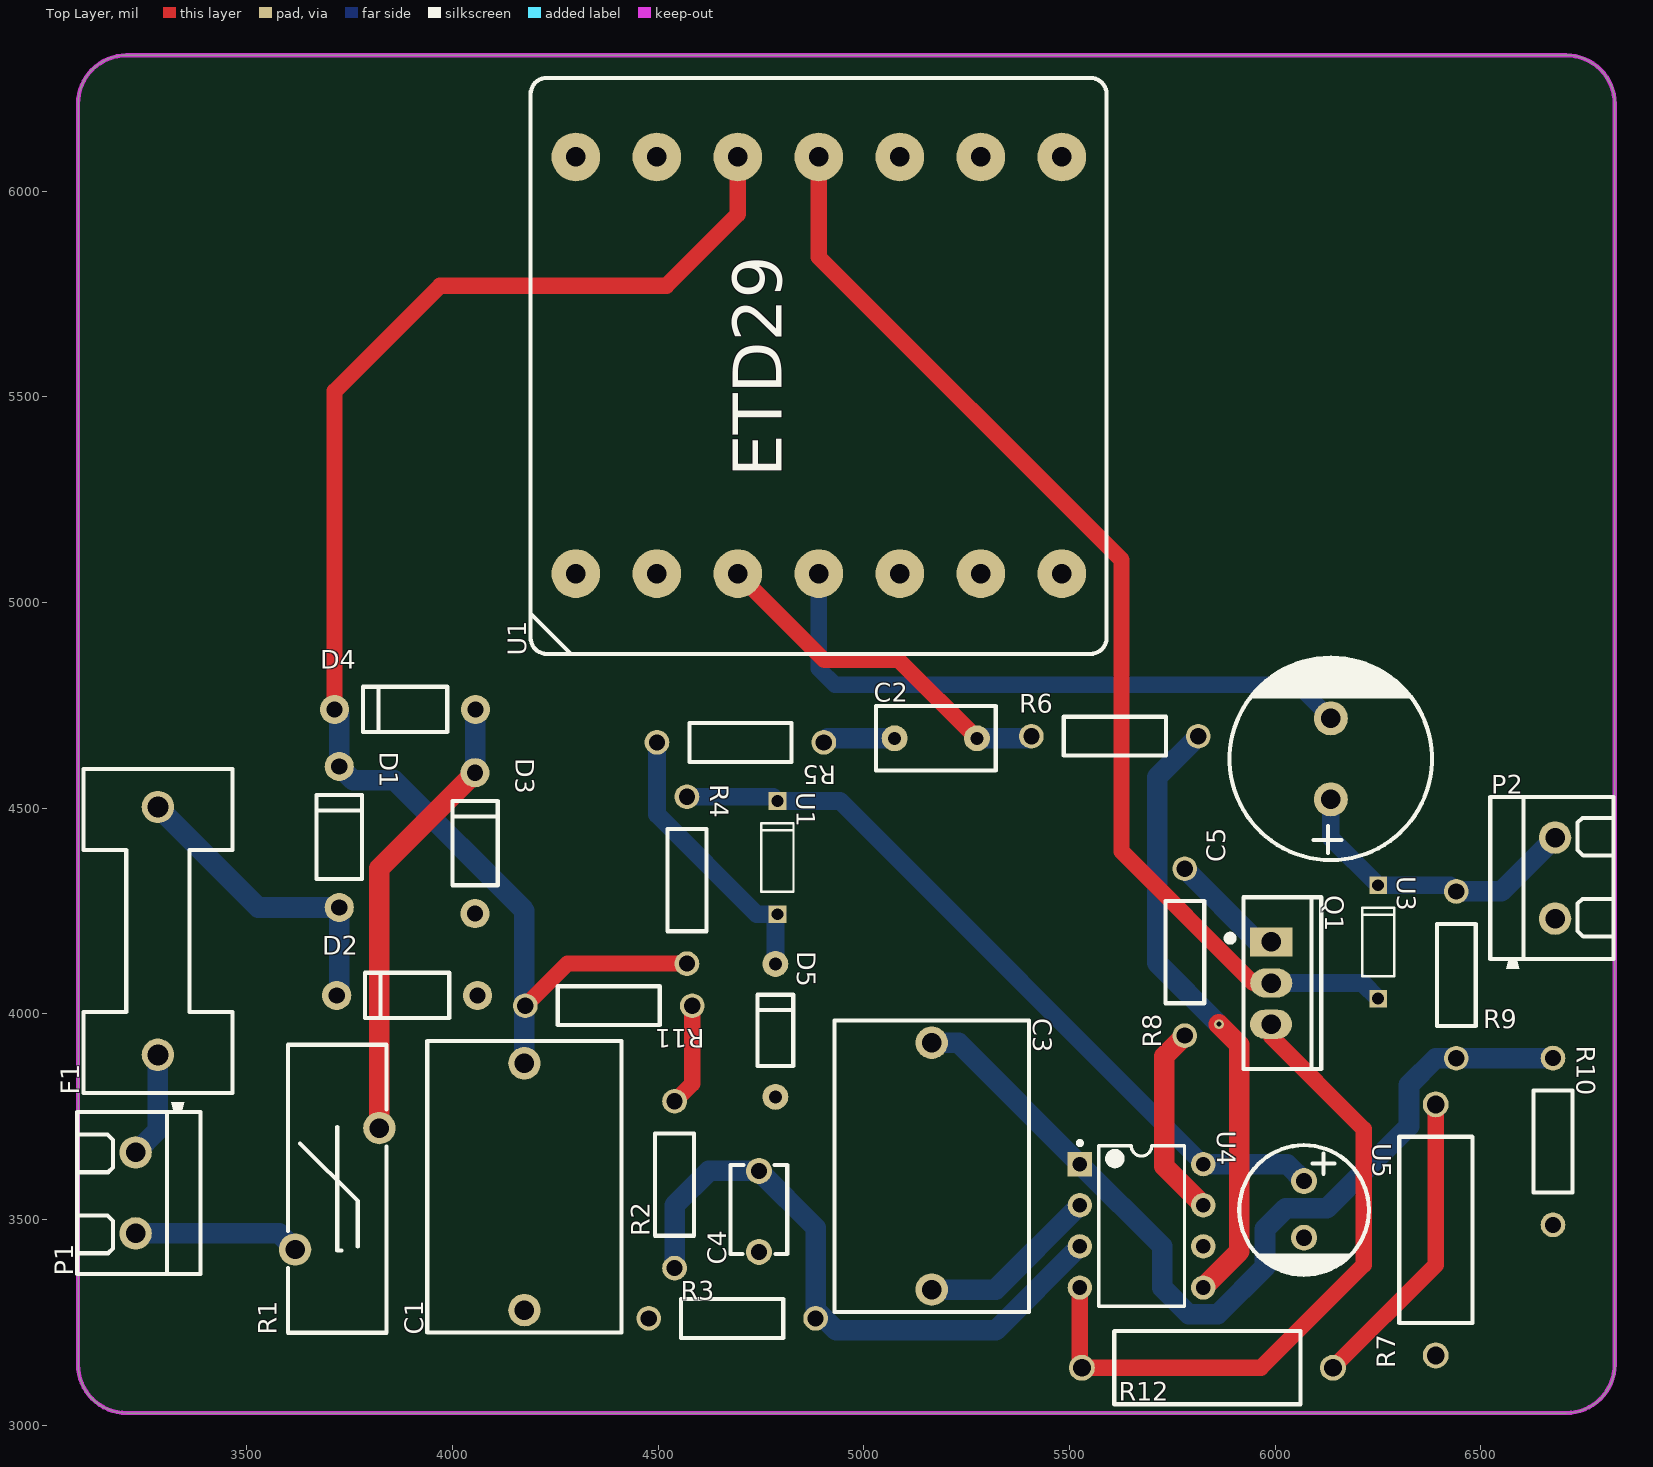
[diagram p0: Top Layer view]
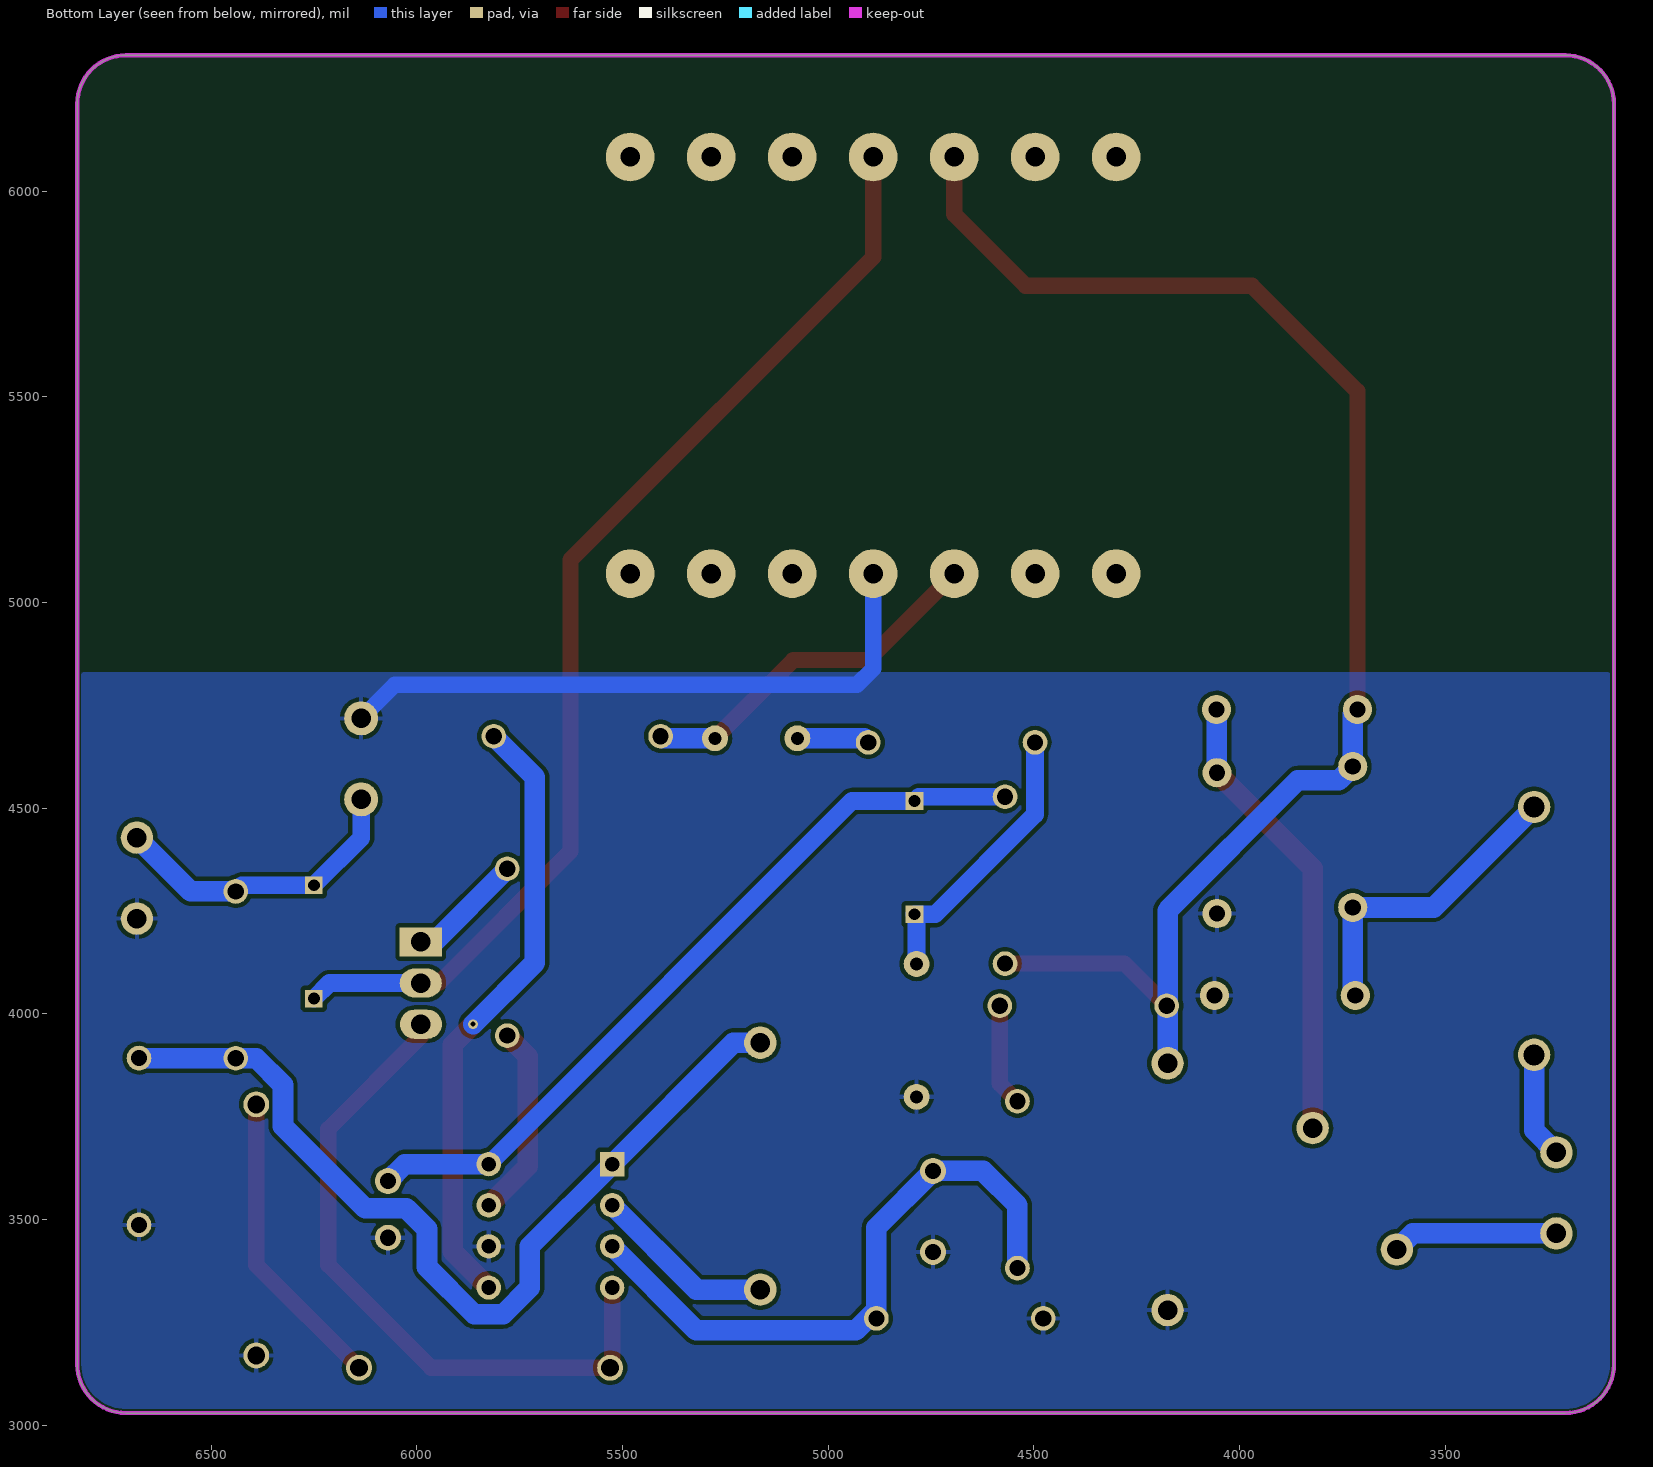
[diagram p1: Bottom Layer view, seen from below]
# Altium PCB MISC89005.pcbdoc
Units mil, origin at the board's own origin, x right, y up, seen from the top; angles counter-clockwise.
Board outline 3735 x 3300 mil, 2 copper layers (Top Layer, Bottom Layer), stack 62.206 mil thick; 31 components, 21 nets, 81 pads, 1 vias.

## Layer stack, top to bottom
Top Solder Mask Layer: solder mask 0.394, Dk 3.3
Top Layer: signal copper 1.379
Dielectric1: surface 59.449, FR4, Dk 4.5
Bottom Layer: signal copper 1.378
Bottom Solder Mask Layer: solder mask 0.394, Dk 3.3

## Board outline
3208.11,6330 ccw(c3208.11,6211.89) 3090,6211.89 3090,3148.11 ccw(c3208.11,3148.11) 3208.11,3030 6706.89,3030 ccw(c6706.89,3148.11) 6825,3148.11 6825,6211.89 ccw(c6706.89,6211.89) 6706.89,6330

## Design rules (kind name [scope] priority, off if disabled: settings)
BoardOutlineClearance copperThickness2oz_1 [All] p2 off: genericclearance=7.99 ignorepadtopadclearanceinfootprint=FALSE except(0: Arc-SplitContinuation Track-SplitContinuation SMDPad-SplitContinuation THPad-SplitContinuation Via-SplitContinuation Fill-SplitContinuation Region-SplitContinuation Poly-SplitContinuation Text-SplitContinuation Hole-SplitContinuation; 5.98: Arc-CutoutEdge Track-CutoutEdge SMDPad-CutoutEdge THPad-CutoutEdge Via-CutoutEdge Text-CutoutEdge; 6.89: Hole-OutlineEdge Hole-CutoutEdge; 10: Poly-OutlineEdge Poly-CutoutEdge; 11.81: Arc-OutlineEdge Track-OutlineEdge SMDPad-OutlineEdge THPad-OutlineEdge Via-OutlineEdge Fill-OutlineEdge Region-OutlineEdge Text-OutlineEdge Fill-CutoutEdge Region-CutoutEdge)
BoardOutlineClearance Plane_innerPlane_1 [All] p4 off: genericclearance=4.02 ignorepadtopadclearanceinfootprint=FALSE except(0: Arc-SplitContinuation Track-SplitContinuation SMDPad-SplitContinuation THPad-SplitContinuation Via-SplitContinuation Fill-SplitContinuation Region-SplitContinuation Poly-SplitContinuation Text-SplitContinuation Hole-SplitContinuation; 5.98: Arc-CutoutEdge Track-CutoutEdge SMDPad-CutoutEdge THPad-CutoutEdge Via-CutoutEdge Text-CutoutEdge; 6.89: Hole-OutlineEdge Hole-CutoutEdge; 10: Poly-OutlineEdge Poly-CutoutEdge; 11.81: Arc-OutlineEdge Track-OutlineEdge SMDPad-OutlineEdge THPad-OutlineEdge Via-OutlineEdge Fill-OutlineEdge Region-OutlineEdge Text-OutlineEdge Fill-CutoutEdge Region-CutoutEdge)
BoardOutlineClearance Copper_copperRegion_1 [All] p6 off: genericclearance=4.02 ignorepadtopadclearanceinfootprint=FALSE except(0: Arc-SplitContinuation Track-SplitContinuation SMDPad-SplitContinuation THPad-SplitContinuation Via-SplitContinuation Fill-SplitContinuation Region-SplitContinuation Poly-SplitContinuation Text-SplitContinuation Hole-SplitContinuation; 5.98: Arc-CutoutEdge Track-CutoutEdge SMDPad-CutoutEdge THPad-CutoutEdge Via-CutoutEdge Text-CutoutEdge; 6.89: Hole-OutlineEdge Hole-CutoutEdge; 10: Poly-OutlineEdge Poly-CutoutEdge; 11.81: Arc-OutlineEdge Track-OutlineEdge SMDPad-OutlineEdge THPad-OutlineEdge Via-OutlineEdge Fill-OutlineEdge Region-OutlineEdge Text-OutlineEdge Fill-CutoutEdge Region-CutoutEdge)
BoardOutlineClearance copperThickness1oz_1 [All] p8: genericclearance=4.02 ignorepadtopadclearanceinfootprint=FALSE except(0: Arc-SplitContinuation Track-SplitContinuation SMDPad-SplitContinuation THPad-SplitContinuation Via-SplitContinuation Fill-SplitContinuation Region-SplitContinuation Poly-SplitContinuation Text-SplitContinuation Hole-SplitContinuation; 5.98: Arc-CutoutEdge Track-CutoutEdge SMDPad-CutoutEdge THPad-CutoutEdge Via-CutoutEdge Text-CutoutEdge; 6.89: Hole-OutlineEdge Hole-CutoutEdge; 10: Poly-OutlineEdge Poly-CutoutEdge; 11.81: Arc-OutlineEdge Track-OutlineEdge SMDPad-OutlineEdge THPad-OutlineEdge Via-OutlineEdge Fill-OutlineEdge Region-OutlineEdge Text-OutlineEdge Fill-CutoutEdge Region-CutoutEdge)
Clearance copperThickness2oz [All] p1 off: gap=7.99 ignorepadtopadclearanceinfootprint=FALSE except(5.98: SMDPad-Track SMDPad-SMDPad THPad-Track SMDPad-THPad THPad-THPad Track-Via SMDPad-Via THPad-Via Via-Via Fill-SMDPad Region-SMDPad Fill-THPad Region-THPad Fill-Via Region-Via Fill-Fill Fill-Region Region-Region Arc-Track Arc-SMDPad Arc-THPad Arc-Via Fill-Arc Region-Arc Arc-Arc Text-Track SMDPad-Text Text-THPad Text-Via Fill-Text Region-Text Arc-Text Text-Text; 6.89: Hole-Track Hole-SMDPad Hole-THPad Hole-Via Fill-Hole Region-Hole Hole-Arc Hole-Text; 10: Poly-Track Poly-SMDPad Poly-THPad Poly-Via Poly-Fill Poly-Region Poly-Poly Poly-Arc Poly-Text Poly-Hole; 11.81: Fill-Track Region-Track)
Clearance Plane_innerPlane [All] p3 off: gap=4.02 ignorepadtopadclearanceinfootprint=FALSE except(5.98: SMDPad-Track SMDPad-SMDPad THPad-Track SMDPad-THPad THPad-THPad Track-Via SMDPad-Via THPad-Via Via-Via Fill-SMDPad Region-SMDPad Fill-THPad Region-THPad Fill-Via Region-Via Fill-Fill Fill-Region Region-Region Arc-Track Arc-SMDPad Arc-THPad Arc-Via Fill-Arc Region-Arc Arc-Arc Text-Track SMDPad-Text Text-THPad Text-Via Fill-Text Region-Text Arc-Text Text-Text; 6.89: Hole-Track Hole-SMDPad Hole-THPad Hole-Via Fill-Hole Region-Hole Hole-Arc Hole-Text; 10: Poly-Track Poly-SMDPad Poly-THPad Poly-Via Poly-Fill Poly-Region Poly-Poly Poly-Arc Poly-Text Poly-Hole; 11.81: Fill-Track Region-Track)
Clearance Copper_copperRegion [All] p5 off: gap=4.02 ignorepadtopadclearanceinfootprint=FALSE except(5.98: SMDPad-Track SMDPad-SMDPad THPad-Track SMDPad-THPad THPad-THPad Track-Via SMDPad-Via THPad-Via Via-Via Fill-SMDPad Region-SMDPad Fill-THPad Region-THPad Fill-Via Region-Via Fill-Fill Fill-Region Region-Region Arc-Track Arc-SMDPad Arc-THPad Arc-Via Fill-Arc Region-Arc Arc-Arc Text-Track SMDPad-Text Text-THPad Text-Via Fill-Text Region-Text Arc-Text Text-Text; 6.89: Hole-Track Hole-SMDPad Hole-THPad Hole-Via Fill-Hole Region-Hole Hole-Arc Hole-Text; 10: Poly-Track Poly-SMDPad Poly-THPad Poly-Via Poly-Fill Poly-Region Poly-Poly Poly-Arc Poly-Text Poly-Hole; 11.81: Fill-Track Region-Track)
Clearance copperThickness1oz [All] p7: gap=4.02 ignorepadtopadclearanceinfootprint=FALSE except(5.98: SMDPad-Track SMDPad-SMDPad THPad-Track SMDPad-THPad THPad-THPad Track-Via SMDPad-Via THPad-Via Via-Via Fill-SMDPad Region-SMDPad Fill-THPad Region-THPad Fill-Via Region-Via Fill-Fill Fill-Region Region-Region Arc-Track Arc-SMDPad Arc-THPad Arc-Via Fill-Arc Region-Arc Arc-Arc Text-Track SMDPad-Text Text-THPad Text-Via Fill-Text Region-Text Arc-Text Text-Text; 6.89: Hole-Track Hole-SMDPad Hole-THPad Hole-Via Fill-Hole Region-Hole Hole-Arc Hole-Text; 10: Poly-Track Poly-SMDPad Poly-THPad Poly-Via Poly-Fill Poly-Region Poly-Poly Poly-Arc Poly-Text Poly-Hole; 11.81: Fill-Track Region-Track)
DiffPairsRouting differentialPair [All] p1: maxlimit=6 minlimit=6 mostfreqgap=6 toplayer_minwidth=5 toplayer_prefwidth=10 toplayer_maxwidth=100 toplayer_mingap=6 toplayer_prefgap=6 toplayer_maxgap=6 bottomlayer_minwidth=5 bottomlayer_prefwidth=10 bottomlayer_maxwidth=100 bottomlayer_mingap=6 bottomlayer_prefgap=6 bottomlayer_maxgap=6 maxuncoupledlength=10
HoleToHoleClearance otherClearance [All] p1: gap=11.81 allowstackedmicrovias=TRUE
Length netLength [All] p1: minlimit=0 maxlimit=0
PasteMaskExpansion pasteMaskExpansion [All] p1: expansion=0
PlaneConnect innerPlane [All] p1: planeconnectstyle=Relief reliefexpansion=20 reliefentries=4 reliefconductorwidth=10 reliefairgap=10
PolygonConnect copperRegion [All] p1: connectstyle=Relief reliefconductorwidth=10 reliefentries=4 polygonreliefangle="90 Angle" airgapwidth=10 via.connectstyle=Relief via.reliefconductorwidth=10 via.reliefentries=4 via.polygonreliefangle="90 Angle" via.airgapwidth=10
RoutingVias viaSize [All] p1: holewidth=12.01 width=24.02 viastyle="Through Hole" minholewidth=11.81 minwidth=19.68 maxholewidth=248.03 maxwidth=393.7
SolderMaskExpansion solderMaskExpansion [IsVia] p1: expansion=-1000 istentingtop=TRUE
SolderMaskExpansion solderMaskExpansion [All] p2: expansion=2.01 istentingtop=FALSE
Width copperThickness2oz_2 [All] p1 off: maxlimit=100 minlimit=8 preferedwidth=10
Width copperThickness1oz_2 [All] p2: maxlimit=100 minlimit=5 preferedwidth=50

## Components (designator, comment, footprint, x,y, rotation, side; value= is the part's Value field where it differs from the comment)
C1 "1uF" CAP-TH_L18.0-W12.0-P15.00-D1.2 4175,3580 r90 top
C2 "12nF" CAP-TH_L7.3-W4.0-P5.00-D0.5 5175,4670 r0 top
C3 "1uF" CAP-TH_L18.0-W12.0-P15.00-D1.2 5165,3630 r270 top
C4 "10nF" CAP-TH_L5.5-W3.5-P5.00-D1.2 4745,3520 r90 top
C5 "47uF" CAP-TH_BD12.5-P5.00-D0.6-FD 6135,4620 r90 top
D1 "" DO_1N4007 3725,4430 r270 top
D2 "" DO_1N4007 3890,4045 r0 top
D3 "" DO_1N4007 4055,4415 r270 top
D4 "" DO_1N4007 3885,4740 r0 top
D5 "1N5248B" DO-35_BD2.0-L4.2-P8.20-D0.5-RD 4785,3960 r270 top
F1 "5*20 fuse holder BF013" FUSE-TH_BF013 3284.09,4201.87 r90 top
P1 "KF301-2P terminal block" CONN-TH_XY301V-A-5.0-2P 3230,3565 r90 top
P2 "KF301-2P terminal block" CONN-TH_XY301V-A-5.0-2P 6680,4330 r270 top
Q1 "STP8NK80Z" TO-220-3_L10.0-W4.5-P2.54-L 5990,4075 r270 top
R1 "WTR15D050MC3BW" RES-TH_L17.5-W6.0-P7.50-D0.8-S5.20 3720,3575 r90 top
R2 "620K" Res_1/4W 4540,3585 r90 top
R3 "10KΩ" Res_1/4W 4680,3260 r0 top
R4 "240kΩ" Res_1/4W 4570,4325 r270 top
R5 "100Ω" Res_1/4W 4700,4660 r180 top
R6 "68kΩ" Res_1/4W 5610,4675 r0 top
R7 "0.22Ω" Res_1W 6390,3475 r90 top
R8 "10Ω" Res_1/4W 5780,4150 r90 top
R9 "998kΩ" Res_1/4W 6440,4095 r270 top
R10 "6.34kΩ" Res_1/4W 6675,3690 r270 top
R11 "620K" Res_1/4W 4380,4020 r180 top
R12 "0.22Ω" Res_1W 5835,3140 r180 top
U1 "1N4150TR" DO-35_BD1.8-L4.1-P7.00-D0.5-RD 4790,4380 r270 top
U1 "" "ETD29 卧式 14脚封装" 4300,5075 r90 top
U3 "1N4150TR" DO-35_BD1.8-L4.1-P7.00-D0.5-RD 6250,4175 r270 top
U4 "L6561" DIP-8_L9.8-W6.6-P2.54-LS7.6-BL 5675,3485 r270 top
U5 "22UF400V" CAP-TH_BD8.0-P3.50-D0.6-FD 6070,3525 r270 top

## Footprints (in the part's own frame and the unit in brackets; to place one, negate y for a bottom-side part, rotate by r counter-clockwise, add the part's x,y. Pads: shape width x height; smd on the part's side, far side on the other; paste and mask are expansions set on the pad)
CAP-TH_BD8.0-P3.50-D0.6-FD [mm]
  round 1.6 hole 1: 1(-1.75,0) 2(1.75,0)
  silkscreen extent -3.96,-4 4.04,4
CAP-TH_BD12.5-P5.00-D0.6-FD [mm]
  round 2.1 hole 1.2 paste+0 mask+0.05: 1(-2.5,0) 2(2.5,0)
  silkscreen extent -6.25,-6.25 6.25,6.25
CAP-TH_L5.5-W3.5-P5.00-D1.2 [mm]
  round 1.6 hole 1: 1(-2.5,0) 2(2.5,0)
  silkscreen extent -2.62,-1.75 2.88,1.75
CAP-TH_L7.3-W4.0-P5.00-D0.5 [mm]
  round 1.6 hole 0.8: 1(-2.54,0) 2(2.54,0)
  silkscreen extent -3.7,-2 3.7,2
CAP-TH_L18.0-W12.0-P15.00-D1.2 [mm]
  round 2 hole 1.2: 1(-7.62,0) 2(7.62,0)
  silkscreen extent -9,-6 9,6
CONN-TH_XY301V-A-5.0-2P [mm]
  round 2 hole 1.2: 1(-2.5,0) 2(2.5,0)
  silkscreen extent -5,-4 5.6,3.6
DIP-8_L9.8-W6.6-P2.54-LS7.6-BL [mm]
  rect 1.5x1.5 hole 0.9: 1(-3.81,-3.81)
  round 1.5 hole 0.9: 2(-1.27,-3.81) 3(1.27,-3.81) 4(3.81,-3.81) 5(3.81,3.81) 6(1.27,3.81) 7(-1.27,3.81) 8(-3.81,3.81)
  silkscreen extent -5.23,-3.93 4.96,2.65
DO-35_BD1.8-L4.1-P7.00-D0.5-RD [mm]
  rect 1.095x1.095 hole 0.73: 1(-3.5,0) 2(3.5,0)
  silkscreen extent -2.11,-0.99 2.11,0.99
DO-35_BD2.0-L4.2-P8.20-D0.5-RD [mm]
  round 1.6 hole 0.8: 1(-4.1,0) 2(4.1,0)
  silkscreen extent -2.2,-1.1 2.2,1.1
DO_1N4007 [mm]
  round 1.8 hole 1 paste+0 mask+0.051: 1(-4.35,0) 2(4.35,0)
  silkscreen extent -2.6,-1.4 2.6,1.4
"ETD29 卧式 14脚封装" [mm]
  round 3 hole 1.2: 1(-0.127,0) 2(-0.127,-5) 3(-0.127,-10) 4(-0.127,-15) 5(-0.127,-20) 6(-0.127,-25) 7(-0.127,-30) 8(25.6,-30) 9(25.6,-25) 10(25.6,-20) 11(25.6,-15) 12(25.6,-10) 13(25.6,-5) 14(25.6,0)
  silkscreen extent -5.08,-32.77 30.48,2.79
FUSE-TH_BF013 [mm]
  round 2 hole 1.3 paste+0 mask+0.05: 1(-7.65,0) 2(7.65,0)
  silkscreen extent -10,-4.6 10,4.6
RES-TH_L17.5-W6.0-P7.50-D0.8-S5.20 [mm]
  round 2 hole 1.2: 1(-3.749,2.6) 2(3.749,-2.6)
  silkscreen extent -8.89,-3.05 8.89,3.05
Res_1/4W [mil]
  round 60 hole 39.37 paste+0 mask+2: 1(-202.76,0) 2(202.76,0)
  silkscreen extent -124,-47 124,47
Res_1W [mm]
  round 1.6 hole 1.1 paste+0 mask+0.051: 1(-7.75,0) 2(7.75,0)
  silkscreen extent -5.75,-2.26 5.75,2.25
TO-220-3_L10.0-W4.5-P2.54-L [mm]
  rect 1.8x2.6 hole 1.2: 1(-2.54,0.005)
  oval 1.8x2.6 hole 1.2: 2(0,0.005)
  oval 1.8x2.6 hole 1.2 copper offset 0,0: 3(2.54,-0.005)
  silkscreen extent -5.3,-2.73 5.3,3.09

## Via types
v1: diameter 24.02, hole 12, Top Layer to Bottom Layer, 1 vias

## Nets (pads, with @x,y where several pads share a name; then routed paths per layer and width w, separated by ;. In a path a pad name is that pad's centre, name@x,y a point inside that pad or via, vN(x,y) a via of type N, cw(c..) or ccw(c..) an arc to the next point about the centre after c; other vN are vias at no path point)
$1N153: F1.1 P1.2 | length 259.7
  Bottom Layer w50: P1.2 3284.09,3717.52 F1.1
$1N187: D1.2 D2.1 F1.2 | length 758.4
  Bottom Layer w50: F1.2 3528.41,4258.74 D1.2 3725,4051.26 D2.1
$1N308: D3.1 D4.2 R1.2 | length 1114.3
  Top Layer w50: R1.2 3822.36,4353.62 D3.1
  Bottom Layer w50: D3.1 4055,4738.74 D4.2
$1N500: P1.1 R1.1 | length 403.9
  Bottom Layer w50: P1.1 3578.46,3466.57 R1.1
$1N614: C4.2 R2.1 R3.2 U4.3 | length 1555.4
  Bottom Layer w50: R2.1 4540,3535 4623.43,3618.43 C4.2 4882.76,3480.66 R3.2@4882.76,3280.66 ; R3.2 R3.2@4882.76,3280.66 ; U4.3 5320.66,3230.66 4932.76,3230.66 R3.2@4882.76,3280.66
$1N691: R4.1 U1.1@4790,4517.8 U4.8 U5.1 | length 1886.8
  Bottom Layer w43.11: R4.1 4780.03,4527.76 4790,4517.8 4942.2,4517.8 U4.8
  Bottom Layer w50: U4.8 6028.9,3635 U5.1
$1N804: D5.1 R5.2 U1.2@4790,4242.2 | length 691.2
  Bottom Layer w43.11: R5.2 4497.24,4484.97 4740,4242.2 4790,4242.2 4785,4237.2 D5.1
$1N890: C2.1 R5.1 | length 176.4
  Bottom Layer w50: R5.1 4912.76,4670 C2.1
$1N951: C2.2 R6.1 U1.3 | length 881.3
  Top Layer w39.37: U1.3 4903.7,4860 5085,4860 C2.2
  Bottom Layer w50: C2.2 5402.24,4670 R6.1
$1N1127: C5.1 P2.1 R9.1 U3.1 | length 746.8
  Bottom Layer w43.11: C5.1 6135,4427.8 U3.1 6424.97,4312.8 R9.1
  Bottom Layer w50: R9.1 6549.34,4297.76 P2.1
$1N1946: R6.2 U4.5 | length 1500.6
  Top Layer w50: U4.5 5912.76,3422.76 5912.76,3925 v1(5862.76,3975)
  Bottom Layer w50: R6.2 5712.76,4575 5712.76,4125 v1(5862.76,3975)
$1N1983: C3.1 R9.2 R10.1 U4.1 | length 2212.2
  Bottom Layer w50: C3.1 5230,3930 U4.1 5725,3435 5725,3335 5789.64,3270.36 5860.36,3270.36 5975,3385 5975,3477.24 6025,3527.24 6125,3527.24 6325,3727.24 6325,3827.24 6390,3892.24 R9.2 6674.48,3892.24 R10.1
$1N1985: C3.2 U4.2 | length 444.9
  Bottom Layer w50: C3.2 5320,3330 U4.2
$1N2304: Q1.3 R12.2 U4.4 | length 1664
  Top Layer w39.37: U4.4 5525,3144.88 R12.2 5965,3140 6215,3390 6215,3720 5989.81,3945.2 Q1.3
$1N2402: R8.1 U4.7 | length 472.3
  Top Layer w50: R8.1 5730,3897.24 5730,3630 U4.7
$1N2516: Q1.1 R8.2 | length 283.8
  Bottom Layer w50: R8.2 5957.76,4175.01 Q1.1
$1N2559: Q1.2 U1.11 U3.2 | length 2764.5
  Top Layer w39.37: U1.11 4890.55,5839.45 5626.34,5103.66 5626.34,4395 5946.34,4075.01 Q1.2
  Bottom Layer w43.11: Q1.2 6212.2,4075.01 U3.2
$1N4051: R2.2 R11.1 | length 250
  Top Layer w39.37: R2.2 4582.76,3830.52 R11.1
$1N4062: C1.2 D1.1 D4.1 R4.2 R11.2 U1.12 | length 3615.7
  Top Layer w39.37: D4.1 3713.74,5513.74 3970,5770 4520,5770 4693.7,5943.7 U1.12 ; R11.2 4279.48,4122.24 R4.2
  Bottom Layer w50: D4.1 3725,4728.74 D1.1 3758.5,4567.76 3858.5,4567.76 4175,4251.26 C1.2
$1N4088: R7.2 R12.1 | length 743.6
  Top Layer w39.37: R12.1 6390,3389.88 R7.2
GND: C1.1 C4.1 C5.2 D2.2 D3.2 D5.2 P2.2 R3.1 R7.1 R10.2 U1.4 U4.6 U5.2 | length 1525.1
  Bottom Layer w39.37: U1.4 4890.55,4839.45 4930,4800 6053.43,4800 C5.2
pads on no net: U1.1@4300,5070 U1.2@4496.85,5070 U1.5 U1.6 U1.7 U1.8 U1.9 U1.10 U1.13 U1.14

## Polygon pours and split planes (outlines as drawn)
GND on Bottom Layer (solid, remove dead copper, pour order 0): 3000,4830 3000,3000 6910,3000 6910,4830

## Keep-outs
Board Outline Layer:
  the board outline again, w10